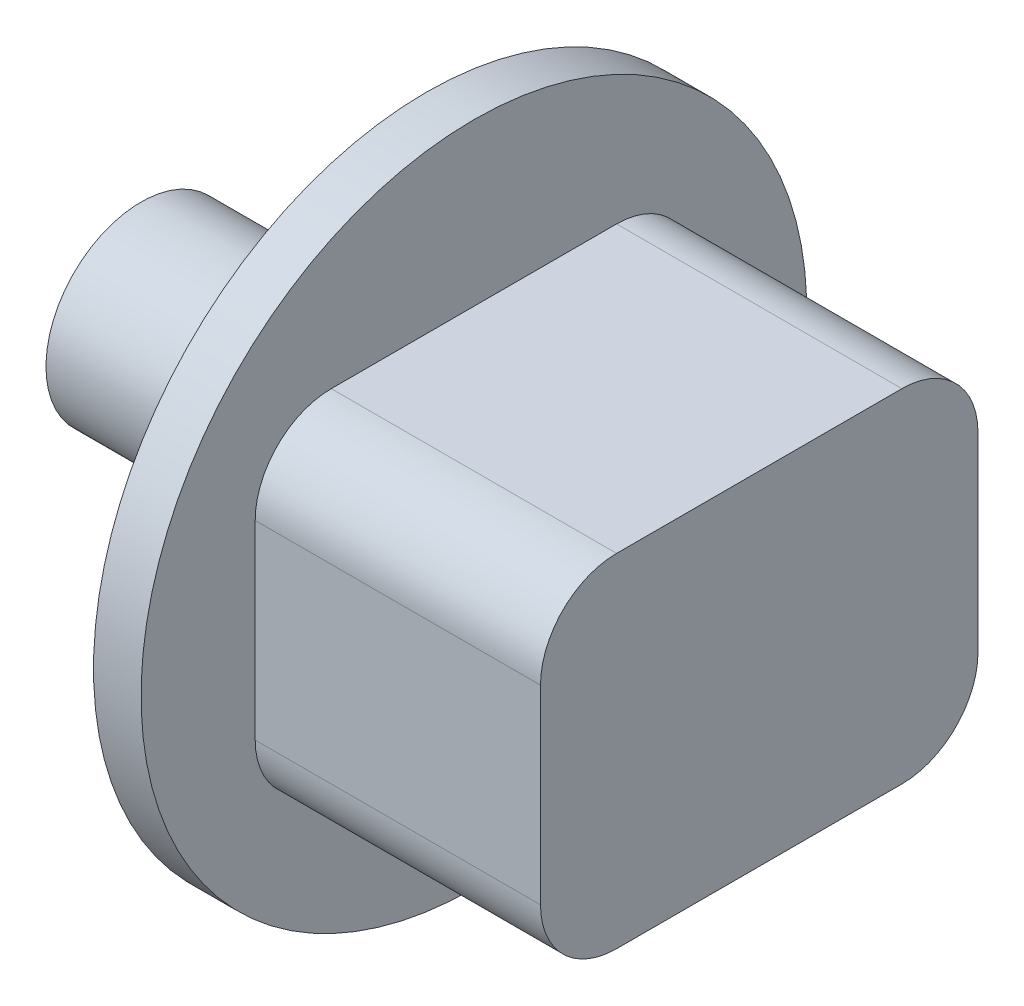
from build123d import *

# Parameters (mm, degrees)
BOSS_EXTRUDE1_DEPTH = 30


with BuildPart() as part:
    # Sketch2 → Boss-Extrude1 (new body)
    with BuildSketch(Plane(origin=(0, 0, 0), x_dir=(0, 0, -1), z_dir=(1, 0, 0))):
        with BuildLine():
            Line((-15, 18), (15, 18))
            ThreePointArc((15, 18), (20.656854249, 15.656854249), (23, 10))
            Line((23, 10), (23, -10))
            ThreePointArc((23, -10), (20.656854249, -15.656854249), (15, -18))
            Line((15, -18), (-15, -18))
            ThreePointArc((-15, -18), (-20.656854249, -15.656854249), (-23, -10))
            Line((-23, -10), (-23, 10))
            ThreePointArc((-23, 10), (-20.656854249, 15.656854249), (-15, 18))
        make_face()
    extrude(amount=-BOSS_EXTRUDE1_DEPTH)

    # Sketch3 → Revolve1 (revolve)
    with BuildSketch(Plane.XY, mode=Mode.PRIVATE) as revolve1_sk:
        Polygon((-30, 0), (-30, 35), (-35, 35), (-35, 10), (-65, 10), (-65, 0), align=None)
    revolve(revolve1_sk.sketch.rotate(Axis((-65, 0, 0), (1, 0, 0)), 180), axis=Axis((-65, 0, 0), (1, 0, 0)))


solid = part.part
